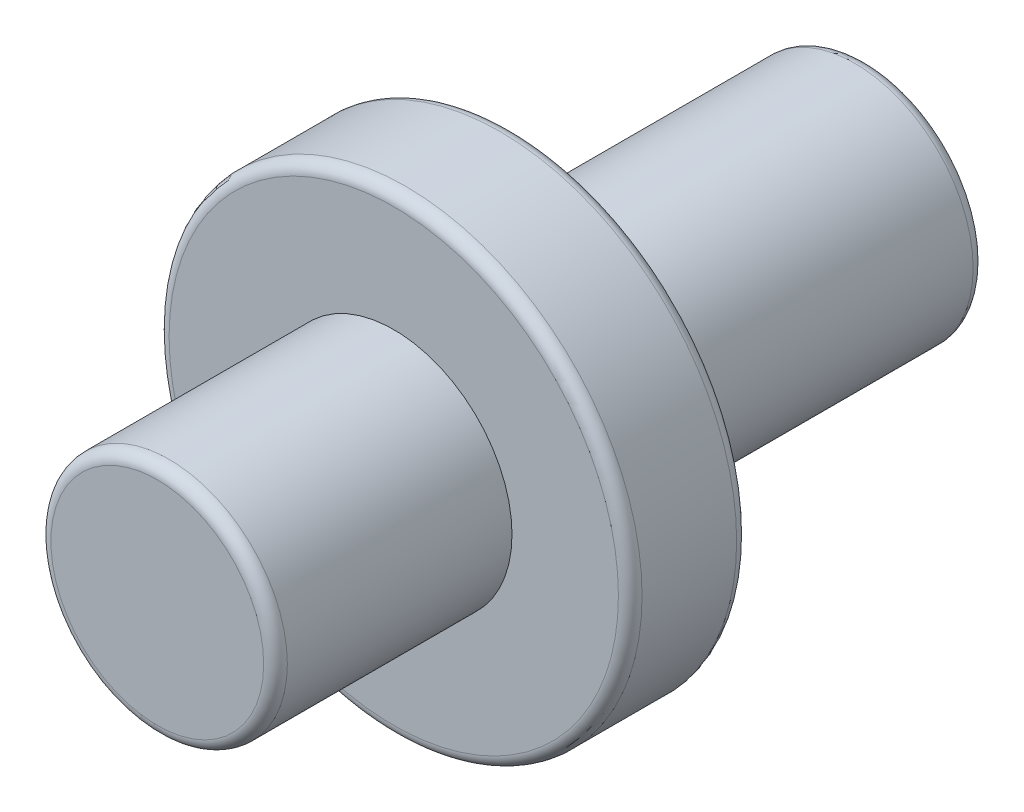
SolidWorks part; units mm, degrees
ref_plane "前视基准面" through (0, 0, 0) normal (0, 0, 1) x (1, 0, 0)
ref_plane "上视基准面" through (0, 0, 0) normal (0, 1, 0) x (1, 0, 0)
ref_plane "右视基准面" through (0, 0, 0) normal (1, 0, 0) x (0, 0, -1)
sketch "草图1" plane through (0, 0, 0) normal (0, 0, 1) x (1, 0, 0)
  circle A0 centre (0, 0) radius 2
  dimension "D1" = 4
extrude "凸台-拉伸1" add sketch "草图1" along normal blind 6
sketch "草图2" plane through (0, 0, 6) normal (0, 0, 1) x (1, 0, 0)
  circle A0 centre (0, 0) radius 4
  dimension "D1" = 8
extrude "凸台-拉伸2" add sketch "草图2" along normal blind 2
sketch "草图3" plane through (0, 0, 8) normal (0, 0, 1) x (1, 0, 0)
  circle A0 centre (0, 0) radius 2
  dimension "D1" = 4
extrude "凸台-拉伸3" add sketch "草图3" along normal blind 4
fillet "圆角1" radius 0.2 2 edges at (2, 0, 0) (2, 0, 12)
fillet "圆角2" radius 0.2 2 edges at (4, 0, 8) (4, 0, 6)
